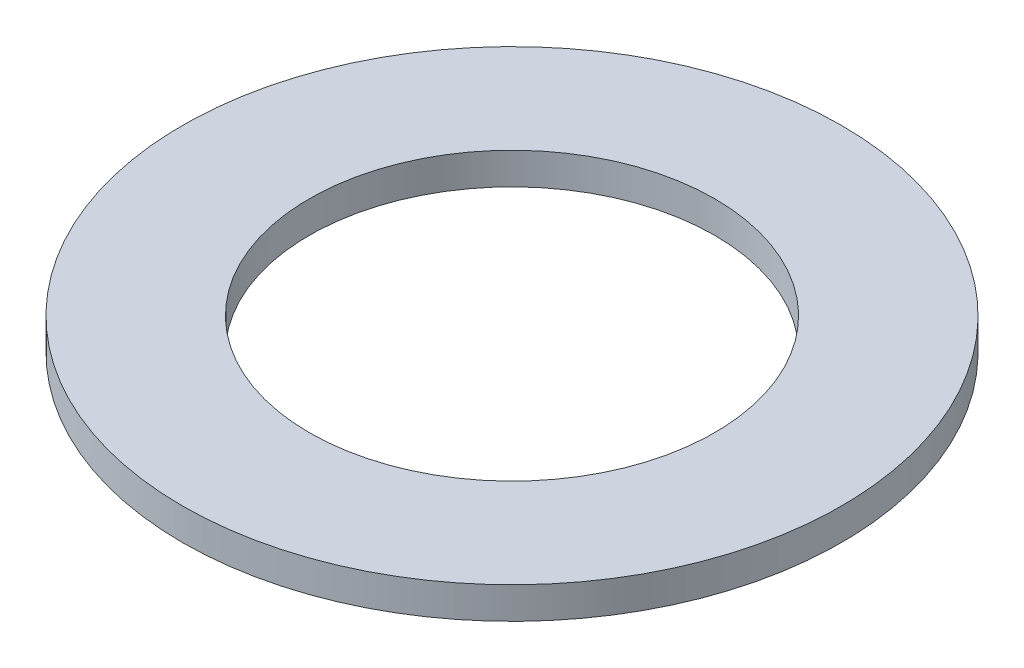
from build123d import *

# Parameters (mm, degrees)
SKETCH_1_R      = 155.82
SKETCH_1_R_2    = 95.82
EXTRUDE_1_DEPTH = 15


with BuildPart() as part:
    # 草图1 → 凸台-拉伸1 (new body)
    with BuildSketch(Plane(origin=(0, 0, 0), x_dir=(1, 0, 0), z_dir=(0, 1, 0))):
        with Locations(Location((0, 0, 0), (0, 0, 270))):
            Circle(SKETCH_1_R)
        with Locations(Location((0, 0, 0), (0, 0, 270))):
            Circle(SKETCH_1_R_2, mode=Mode.SUBTRACT)
    extrude(amount=EXTRUDE_1_DEPTH)


solid = part.part
